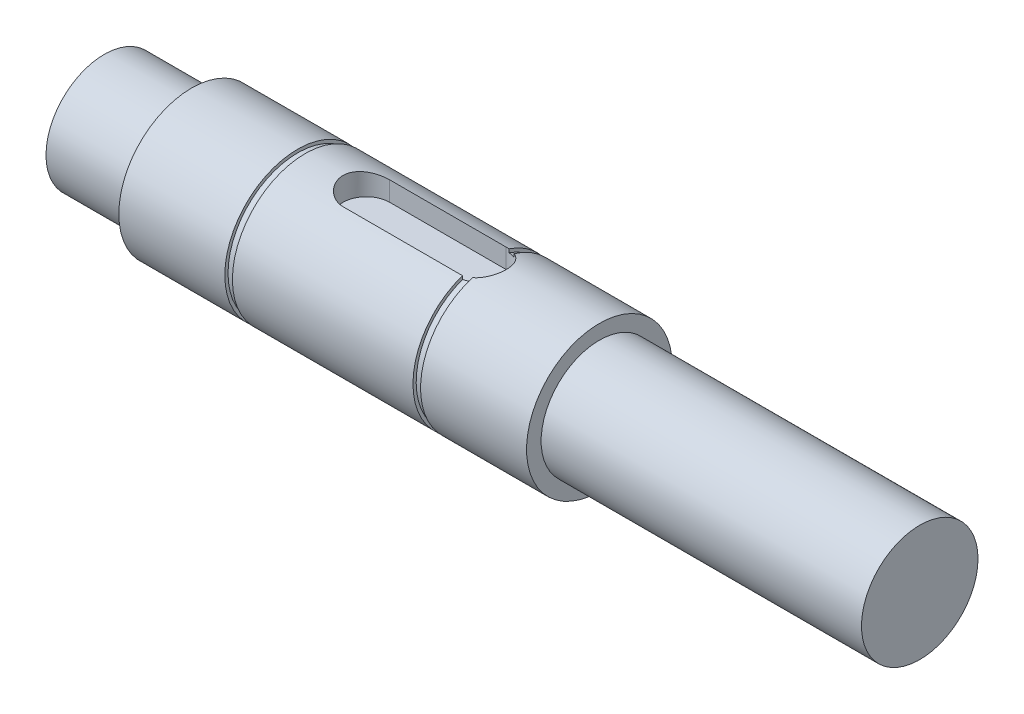
SolidWorks part; units mm, degrees
ref_plane "前视基准面" through (0, 0, 0) normal (0, 0, 1) x (1, 0, 0)
ref_plane "上视基准面" through (0, 0, 0) normal (0, 1, 0) x (1, 0, 0)
ref_plane "右视基准面" through (0, 0, 0) normal (1, 0, 0) x (0, 0, -1)
sketch "草图1" plane through (0, 0, 0) normal (1, 0, 0) x (0, 0, -1)
  circle A0 centre (0, 0) radius 12.5
  dimension "D1" = 25
extrude "凸台-拉伸1" add sketch "草图1" along normal mid plane 70
sketch "草图3" plane through (35, 0, 0) normal (1, 0, 0) x (0, 0, -1)
  circle A0 centre (0, 0) radius 10
  dimension "D1" = 20
extrude "凸台-拉伸3" add sketch "草图3" along normal blind 55
ref_plane "基准面1" through (0, 500, 0) normal (0, 1, 0) x (1, 0, 0)
sketch "草图4" plane through (0, 0, 0) normal (0, 1, 0) x (1, 0, 0)
  line L0 (35, 12.5) -> (-35, 12.5) construction
  line L1 (-16.8, 12.5) -> (-15.5, 12.5)
  line L2 (-16.8, 12.5) -> (-16.8, 11.95)
  line L3 (-16.8, 11.95) -> (-15.5, 11.95)
  line L4 (-15.5, 12.5) -> (-15.5, 11.95)
  line L5 (0, 0) -> (0, 24.3288) construction
  line L6 (15.5, 12.5) -> (16.8, 12.5)
  line L7 (15.5, 12.5) -> (15.5, 11.95)
  line L8 (15.5, 11.95) -> (16.8, 11.95)
  line L9 (16.8, 12.5) -> (16.8, 11.95)
  line L10 (0, 0) -> (0.0569, 0) construction
  line L11 (35, -12.5) -> (35, 12.5) construction
  dimension "D1" = 11.95
  dimension "D2" = 1.3
  dimension "D3" = 31
  dimension "D4" = 35
revolve "切除-旋转1" cut sketch "草图4" angle 360 about L10
ref_plane "基准面2" through (0, 8.5, 0) normal (0, 1, 0) x (1, 0, 0)
sketch "草图5" plane through (0, 8.5, 0) normal (0, 1, 0) x (1, 0, 0)
  line L0 (-5, 0) -> (15, 0) construction
  line L1 (-5, 4) -> (15, 4)
  line L2 (-5, -4) -> (15, -4)
  line L3 (35, -10) -> (35, 10) construction
  arc A0 (-5, 4) -> (-5, -4) centre (-5, 0) ccw
  arc A1 (15, -4) -> (15, 4) centre (15, 0) ccw
  point P3 (5, 0)
  dimension "D1" = 20
  dimension "D2" = 8
  dimension "D3" = 30
extrude "切除-拉伸1" cut sketch "草图5" along normal through all
sketch "草图6" plane through (-35, 0, 0) normal (-1, 0, 0) x (0, 0, 1)
  circle A0 centre (0, 0) radius 10
  dimension "D1" = 20
extrude "凸台-拉伸4" add sketch "草图6" along normal blind 15
